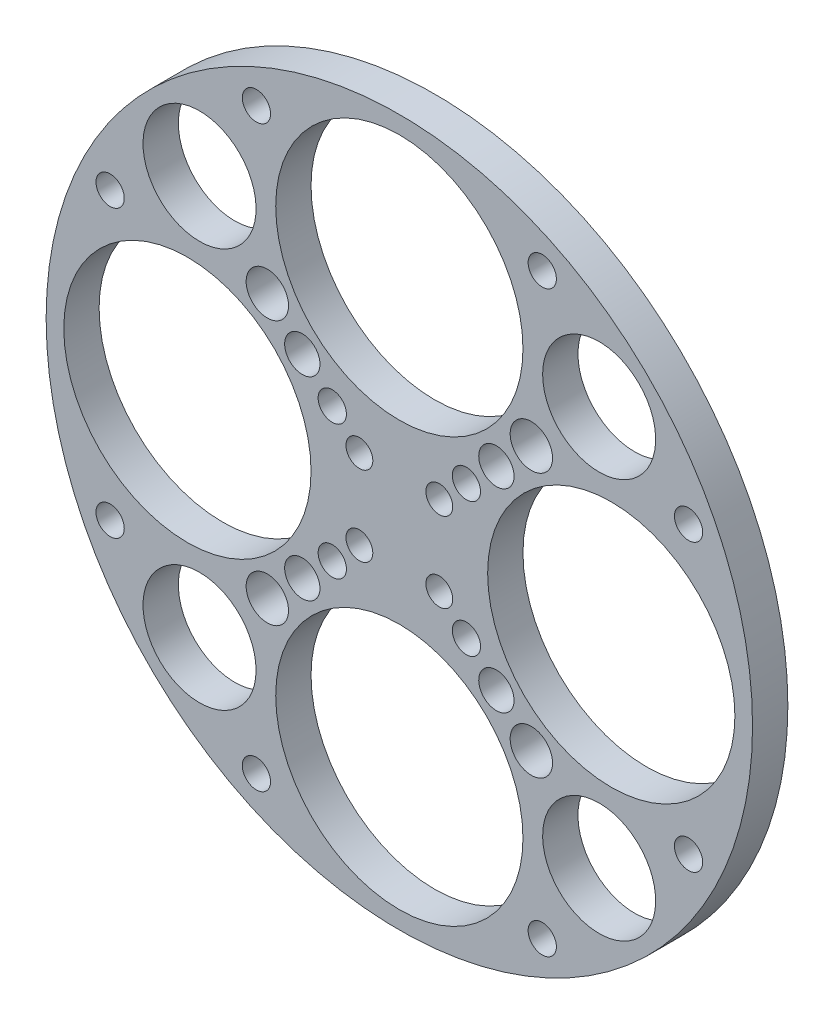
from build123d import *

# Parameters (mm, degrees)
SKETCH1_R           = 50
BOSS_EXTRUDE1_DEPTH = 5
SKETCH2_R           = 1.9
CUT_EXTRUDE1_DEPTH  = 71.887234394
CIRPATTERN1_COUNT   = 4
SKETCH3_R           = 17.5
CUT_EXTRUDE2_DEPTH  = 71.887234394
CIRPATTERN2_COUNT   = 4
SKETCH4_R           = 8
SKETCH4_R_2         = 3
SKETCH4_R_3         = 2.5
SKETCH4_R_4         = 2
CUT_EXTRUDE3_DEPTH  = 71.887234394
CIRPATTERN3_COUNT   = 4


with BuildPart() as part:
    # Sketch1 → Boss-Extrude1 (new body)
    with BuildSketch(Plane.XY):
        Circle(SKETCH1_R)
    extrude(amount=BOSS_EXTRUDE1_DEPTH)

    # Sketch2 → Cut-Extrude1 (cut, through all)
    with BuildSketch(Plane(origin=(0, 0, 0), x_dir=(-1, 0, 0), z_dir=(0, 0, -1))):
        with Locations((-5.656854249, 5.656854249)):
            Circle(SKETCH2_R)
    cut_extrude1 = extrude(amount=-CUT_EXTRUDE1_DEPTH, mode=Mode.SUBTRACT)

    # CirPattern1: Cut-Extrude1 ×4 about axis
    cirpattern1_axis = Axis((0, 0, 0), (0, 0, 1))
    for i in range(1, CIRPATTERN1_COUNT):
        add(cut_extrude1.rotate(cirpattern1_axis, i * 360 / CIRPATTERN1_COUNT), mode=Mode.SUBTRACT)

    # Sketch3 → Cut-Extrude2 (cut, through all)
    with BuildSketch(Plane(origin=(0, 0, 0), x_dir=(-1, 0, 0), z_dir=(0, 0, -1))):
        with Locations((0, 30)):
            Circle(SKETCH3_R)
    cut_extrude2 = extrude(amount=-CUT_EXTRUDE2_DEPTH, mode=Mode.SUBTRACT)

    # CirPattern2: Cut-Extrude2 ×4 about axis
    cirpattern2_axis = Axis((0, 0, 0), (0, 0, 1))
    for i in range(1, CIRPATTERN2_COUNT):
        add(cut_extrude2.rotate(cirpattern2_axis, i * 360 / CIRPATTERN2_COUNT), mode=Mode.SUBTRACT)

    # Sketch4 → Cut-Extrude3 (cut, through all)
    with BuildSketch(Plane(origin=(0, 0, 0), x_dir=(-1, 0, 0), z_dir=(0, 0, -1))):
        with Locations((-28.284271247, 28.284271247)):
            Circle(SKETCH4_R)
        with Locations((-18.686291501, 18.686291501)):
            Circle(SKETCH4_R_2)
        with Locations((-13.736544033, 13.736544033)):
            Circle(SKETCH4_R_3)
        with Locations((-9.493903346, 9.493903346)):
            Circle(SKETCH4_R_4)
        with Locations((-20.231783609, 40.939603832)):
            Circle(SKETCH4_R_4)
        with Locations((-40.939603832, 20.231783609)):
            Circle(SKETCH4_R_4)
    cut_extrude3 = extrude(amount=-CUT_EXTRUDE3_DEPTH, mode=Mode.SUBTRACT)

    # CirPattern3: Cut-Extrude3 ×4 about axis
    cirpattern3_axis = Axis((0, 0, 0), (0, 0, 1))
    for i in range(1, CIRPATTERN3_COUNT):
        add(cut_extrude3.rotate(cirpattern3_axis, i * 360 / CIRPATTERN3_COUNT), mode=Mode.SUBTRACT)


solid = part.part
